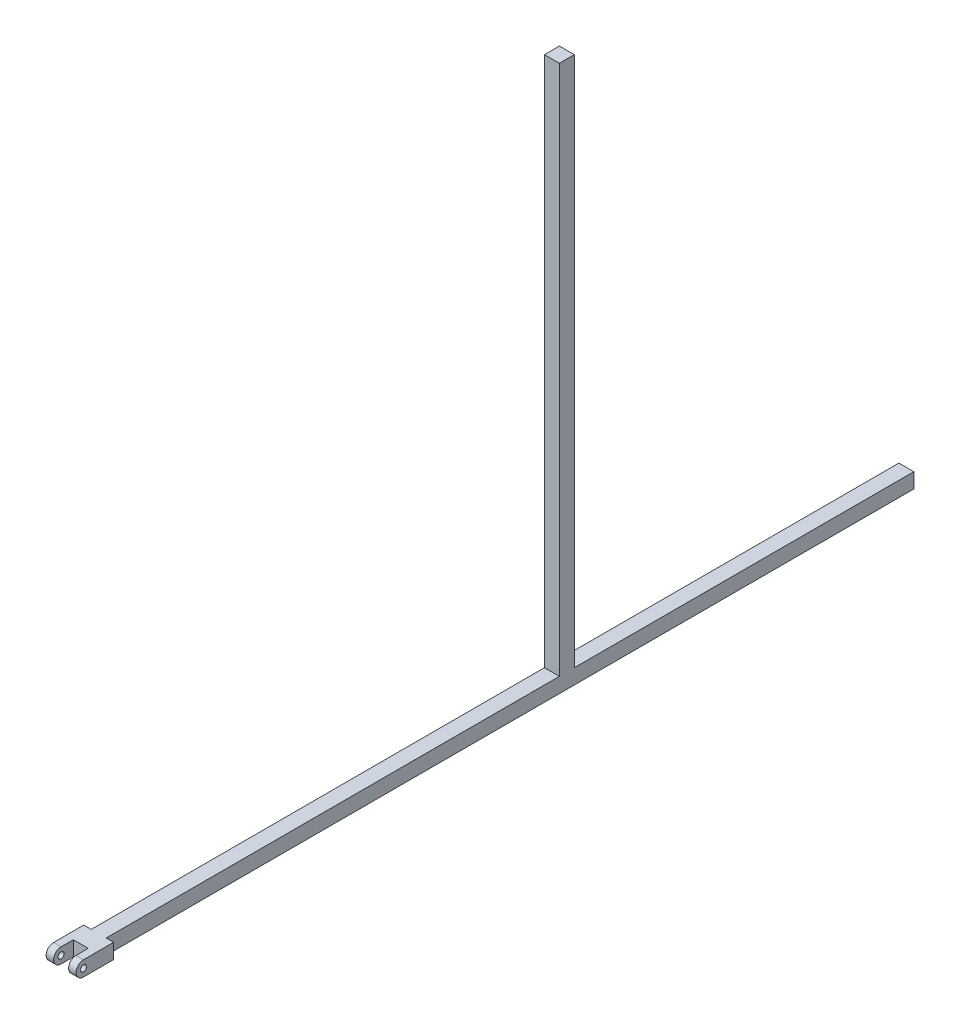
SolidWorks part; units mm, degrees
ref_plane "Front Plane" through (0, 0, 0) normal (0, 0, 1) x (1, 0, 0)
ref_plane "Top Plane" through (0, 0, 0) normal (0, 1, 0) x (1, 0, 0)
ref_plane "Right Plane" through (0, 0, 0) normal (1, 0, 0) x (0, 0, -1)
other "Configuration Table"
sketch "Sketch1" plane through (0, 0, 0) normal (0, 0, 1) x (1, 0, 0)
  line L1 (-2.5, 2.5) -> (2.5, 2.5)
  line L2 (-2.5, 2.5) -> (-2.5, -2.5)
  line L3 (-2.5, -2.5) -> (2.5, -2.5)
  line L4 (2.5, 2.5) -> (2.5, -2.5)
  line L5 (-2.5, 2.5) -> (2.5, -2.5) construction
  line L6 (-2.5, -2.5) -> (2.5, 2.5) construction
  point P0 (0, 0)
  dimension "D1" = 5
  dimension "D2" = 5
extrude "Boss-Extrude1" add sketch "Sketch1" along normal blind 270
sketch "Sketch2" plane through (0, 0, 270) normal (0, 0, 1) x (1, 0, 0)
  line L1 (-5, 2.5) -> (5, 2.5)
  line L2 (-5, 2.5) -> (-5, -2.5)
  line L3 (-5, -2.5) -> (5, -2.5)
  line L4 (5, 2.5) -> (5, -2.5)
  line L5 (-5, 2.5) -> (5, -2.5) construction
  line L6 (-5, -2.5) -> (5, 2.5) construction
  point P0 (0, 0)
  dimension "D1" = 10
  dimension "D2" = 5
extrude "Boss-Extrude2" add sketch "Sketch2" along normal blind 18
sketch "Sketch3" plane through (0, 0, 288) normal (0, 0, 1) x (1, 0, 0)
  line L1 (-2.5, 9.6791) -> (2.5, 9.6791)
  line L2 (-2.5, 9.6791) -> (-2.5, -9.6791)
  line L3 (-2.5, -9.6791) -> (2.5, -9.6791)
  line L4 (2.5, 9.6791) -> (2.5, -9.6791)
  line L5 (-2.5, 9.6791) -> (2.5, -9.6791) construction
  line L6 (-2.5, -9.6791) -> (2.5, 9.6791) construction
  point P0 (0, 0)
  dimension "D1" = 5
extrude "Cut-Extrude1" cut sketch "Sketch3" against normal blind 12
sketch "Sketch4" plane through (5, 0, 0) normal (1, 0, 0) x (0, 0, -1)
  line L0 (-280.0767, 2.5) -> (-280.0767, 12.0985)
  line L1 (-280.0767, 12.0985) -> (-285.8812, 12.0985)
  line L2 (-285.8812, 12.0985) -> (-318.8272, -19.1422)
  line L3 (-318.8272, -19.1422) -> (-280.0767, -2.5)
  line L4 (-288, -2.5) -> (-288, 2.5) construction
  circle A0 centre (-280.0767, 0) radius 1
  arc A1 (-280.0767, 2.5) -> (-280.0767, -2.5) centre (-280.0767, 0) ccw
  dimension "D1" = 2
  dimension "D2" = 5
  dimension "D3" = 7.9233
extrude "Cut-Extrude2" cut sketch "Sketch4" against normal through all both and the other way through all
sketch "Sketch5" plane through (0, 0, 0) normal (0, 1, 0) x (1, 0, 0)
  line L1 (2.5, -270) -> (2.5, 0) construction
  line L2 (-2.5, -113.5) -> (2.5, -113.5)
  line L3 (-2.5, -113.5) -> (-2.5, -118.5)
  line L4 (-2.5, -118.5) -> (2.5, -118.5)
  line L5 (2.5, -113.5) -> (2.5, -118.5)
  line L6 (-2.5, -113.5) -> (2.5, -118.5) construction
  line L7 (-2.5, -118.5) -> (2.5, -113.5) construction
  point P0 (0, -116)
  dimension "D1" = 5
  dimension "D2" = 116
  dimension "D3" = 5
extrude "Boss-Extrude3" add sketch "Sketch5" along normal blind 180
sketch "Sketch6" plane through (-2.5, 0, 0) normal (1, 0, 0) x (0, 0, -1)
  line L0 (-280.0767, 0) -> (-279.0767, 0) construction
  circle A0 centre (-280.0767, 0) radius 1 construction
